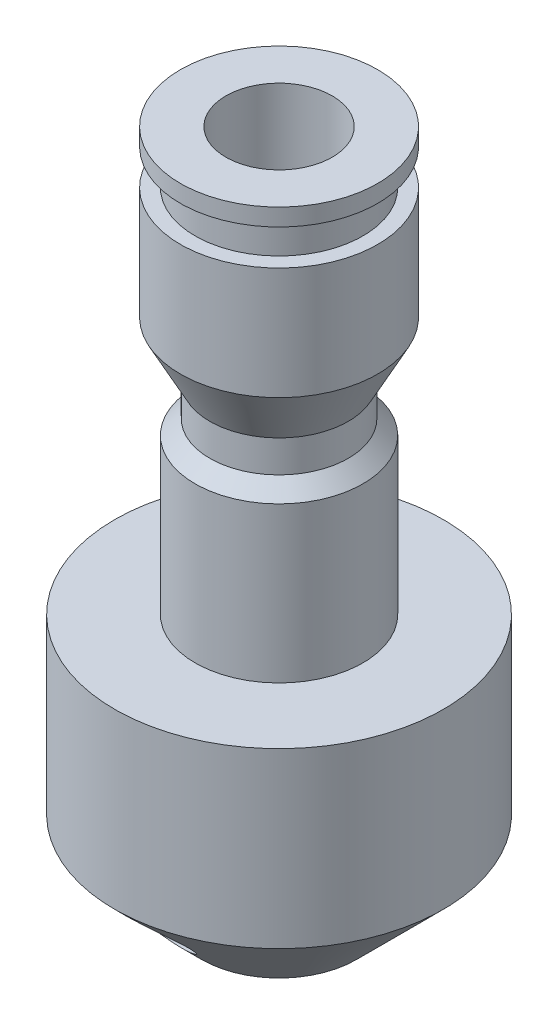
from build123d import *

# Parameters (mm, degrees)
SKETCH3_R          = 2.75
CUT_EXTRUDE2_DEPTH = 4
SKETCH4_R          = 4
CUT_EXTRUDE3_DEPTH = 10
SKETCH5_W          = 5.699016122
SKETCH5_H          = 1.5


with BuildPart() as part:
    # Sketch1 → Revolve1 (revolve)
    with BuildSketch(Plane.XY):
        Polygon((-8.5, -6.487039895), (-8.5, -15.445084434), (-4, -19.945084434), (0, -19.945084434), (0, 12.633854157), (0, 15.364763468), (-5.101647841, 15.364763468), (-5.101647841, 14.4706398), (-4.341150579, 14.4706398), (-4.341150579, 12.633854157), (-5.101647841, 12.633854157), (-5.101647841, 6.827224241), (-3.580653318, 3.948464428), (-3.580653318, 2.293177536), (-4.341150579, 1.532680274), (-4.341150579, -6.487039895), align=None)
    revolve(axis=Axis((0, 12.633854157, 0), (0, -1, 0)))

    # Sketch3 → Cut-Extrude2 (cut)
    with BuildSketch(Plane(origin=(0, 15.364763468, 0), x_dir=(1, 0, 0), z_dir=(0, 1, 0))):
        with Locations(Location((0, 0, 0), (0, 0, 180))):
            Circle(SKETCH3_R)
    extrude(amount=-CUT_EXTRUDE2_DEPTH, mode=Mode.SUBTRACT)

    # Sketch4 → Cut-Extrude3 (cut)
    with BuildSketch(Plane.XZ.offset(19.945084434)):
        Circle(SKETCH4_R)
    extrude(amount=-CUT_EXTRUDE3_DEPTH, mode=Mode.SUBTRACT)

    # Sketch5 → Cut-Revolve1 (revolve, cut)
    with BuildSketch(Plane(origin=(0, 0, 0), x_dir=(0, 0, -1), z_dir=(1, 0, 0)), mode=Mode.PRIVATE) as cut_revolve1_sk:
        with Locations((6.332308204, -16.695084434)):
            Rectangle(SKETCH5_W, SKETCH5_H)
    cut_revolve1 = revolve(cut_revolve1_sk.sketch.rotate(Axis((0, -17.445084434, -3.482800143), (0, 0, -1)), 90), axis=Axis((0, -17.445084434, -3.482800143), (0, 0, -1)), mode=Mode.SUBTRACT)

    # Mirror1: Cut-Revolve1 across plane
    add(cut_revolve1.mirror(Plane.XY), mode=Mode.SUBTRACT)


solid = part.part
